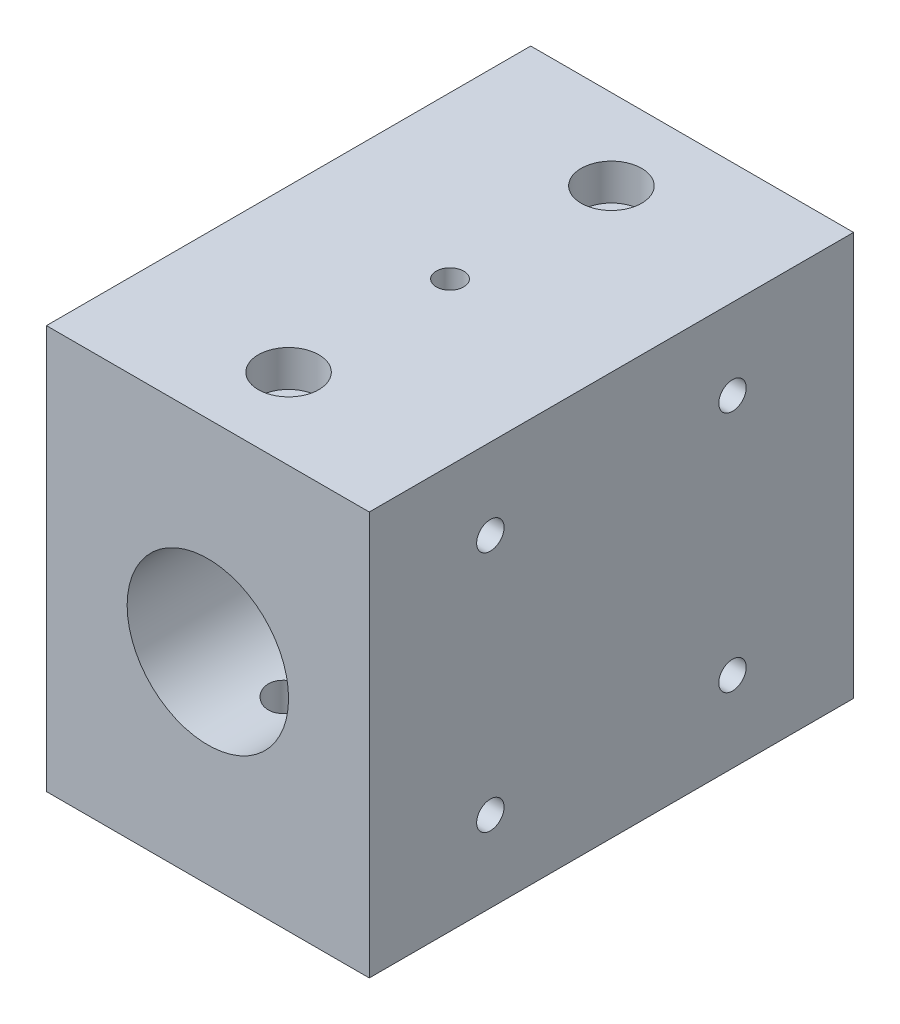
SolidWorks part; units mm, degrees
material "45#"
ref_plane "Front Plane" through (0, 0, 0) normal (0, 0, 1) x (1, 0, 0)
ref_plane "Top Plane" through (0, 0, 0) normal (0, 1, 0) x (1, 0, 0)
ref_plane "Right Plane" through (0, 0, 0) normal (1, 0, 0) x (0, 0, -1)
sketch "Sketch1" plane through (0, 0, 0) normal (0, 0, 1) x (1, 0, 0)
  line L5 (-40, 50) -> (40, 50)
  line L6 (-40, 50) -> (-40, -50)
  line L7 (-40, -50) -> (40, -50)
  line L8 (40, 50) -> (40, -50)
  line L9 (-40, 50) -> (40, -50) construction
  line L10 (-40, -50) -> (40, 50) construction
  point P0 (0, 0)
  dimension "D1" = 80
  dimension "D2" = 100
extrude "Boss-Extrude1" add sketch "Sketch1" along normal blind 120
sketch "Sketch2" plane through (0, 0, 120) normal (0, 0, 1) x (1, 0, 0)
  circle A0 centre (0, 0) radius 20
  dimension "D1" = 40
extrude "Cut-Extrude1" cut sketch "Sketch2" against normal through all
sketch "Sketch15" plane through (0, 0, 0) normal (0, 0, -1) x (-1, 0, 0)
  line L0 (-17.8606, 9) -> (-17.8606, -9)
  line L1 (0, 0) -> (0, -20) construction
  line L3 (0, 0) -> (20, 0) construction
  line L5 (17.8606, 9) -> (17.8606, -9)
  line L6 (-9, 17.8606) -> (9, 17.8606)
  line L7 (-9, -17.8606) -> (9, -17.8606)
  arc A0 (-9, -17.8606) -> (9, -17.8606) centre (0, 0) ccw
  circle A1 centre (0, 0) radius 20 construction
  arc A2 (-17.8606, 9) -> (-17.8606, -9) centre (0, 0) ccw
  arc A3 (9, 17.8606) -> (-9, 17.8606) centre (0, 0) ccw
  arc A4 (17.8606, -9) -> (17.8606, 9) centre (0, 0) ccw
  dimension "D1" = 18
extrude "Boss-Extrude2" [suppressed] add sketch "Sketch15" against normal blind 120
hole_wizard "Hole Size (based on) hex socket cap screw type 2" positions "Sketch3" profile "Sketch4" counterbore size "M8" standard "GB"
sketch "Sketch3" plane through (0, 50, 0) normal (0, 1, 0) x (1, 0, 0)
  line L0 (0, 0) -> (0, -20) construction
  point P0 (0, -20)
  point P2 (0, -100)
  dimension "D1" = 20
  dimension "D2" = 80
sketch "Sketch4" plane through (0, 50, 20) normal (1, 0, 0) x (0, 0, 1)
  line L0 (0, 0) -> (0, 38.0043)
  line L1 (0, 38.0043) -> (5, 35)
  line L2 (5, 35) -> (5, 9)
  line L3 (5, 9) -> (7.5, 9)
  line L4 (7.5, 9) -> (7.5, 0)
  line L5 (7.5, 0) -> (0, 0)
  line L10 (0, 38.0043) -> (-5, 35) construction
  line L11 (0, -6.35) -> (0, 107.95) construction
  dimension "孔直径" = 10
  dimension "孔深度" = 35
  dimension "柱形沉头孔直径" = 15
  dimension "柱形沉头孔深度" = 9
  dimension "导头角度" = 118
hole_wizard "打孔尺寸(%根据)内六角圆柱头螺钉的类型2" positions "Sketch6" profile "Sketch7" counterbore size "M8" standard "GB"
sketch "Sketch6" plane through (0, -50, 0) normal (0, -1, 0) x (-1, 0, 0)
  point P0 (0, -20)
  point P3 (0, -100)
sketch "Sketch7" plane through (0, -50, 20) normal (1, 0, 0) x (0, 0, -1)
  line L0 (0, 0) -> (0, 53.0043)
  line L1 (0, 53.0043) -> (5, 50)
  line L2 (5, 50) -> (5, 9)
  line L3 (5, 9) -> (7.5, 9)
  line L4 (7.5, 9) -> (7.5, 0)
  line L5 (7.5, 0) -> (0, 0)
  line L10 (0, 53.0043) -> (-5, 50) construction
  line L11 (0, -6.35) -> (0, 107.95) construction
  dimension "孔直径" = 10
  dimension "孔深度" = 50
  dimension "柱形沉头孔直径" = 15
  dimension "柱形沉头孔深度" = 9
  dimension "导头角度" = 118
hole_wizard "M8 Tapped Hole1" positions "Sketch8" profile "Sketch9" tap size "M8" standard "GB"
sketch "Sketch8" plane through (-40, 0, 0) normal (-1, 0, 0) x (0, 0, 1)
  line L0 (0, 0) -> (41.0233, 0) construction
  line L2 (60, 50) -> (60, 32.9358) construction
  line L3 (120, 50) -> (0, 50) construction
  point P0 (30, 30)
  point P2 (90, 30)
  point P4 (90, -30)
  point P6 (30, -30)
  dimension "D1" = 60
  dimension "D2" = 60
sketch "Sketch9" plane through (-40, 30, 30) normal (0, 1, 0) x (0, 0, 1)
  line L0 (0, 0) -> (0, 32.0429)
  line L1 (0, 32.0429) -> (3.4, 30)
  line L2 (3.4, 30) -> (3.4, 0)
  line L5 (3.4, 0) -> (0, 0)
  line L10 (0, 32.0429) -> (-3.4, 30) construction
  line L11 (0, -6.35) -> (0, 107.95) construction
  dimension "螺纹孔钻头直径" = 6.8
  dimension "螺纹孔钻头深度" = 30
  dimension "导头角度" = 118
cosmetic thread "Cosmetic Thread1" parameters "D1"=16, "D2"=8
cosmetic thread "Cosmetic Thread2" parameters "D1"=16, "D2"=8
cosmetic thread "Cosmetic Thread3" parameters "D1"=16, "D2"=8
cosmetic thread "Cosmetic Thread4" parameters "D1"=16, "D2"=8
hole_wizard "M8 Tapped Hole2" positions "Sketch10" profile "Sketch11" tap size "M8" standard "GB"
sketch "Sketch10" plane through (40, 0, 0) normal (1, 0, 0) x (0, 0, -1)
  point P0 (-90, 30)
  point P2 (-30, 30)
  point P5 (-30, -30)
  point P8 (-90, -30)
sketch "Sketch11" plane through (40, 30, 90) normal (0, 1, 0) x (0, 0, -1)
  line L0 (0, 0) -> (0, 32.0429)
  line L1 (0, 32.0429) -> (3.4, 30)
  line L2 (3.4, 30) -> (3.4, 0)
  line L5 (3.4, 0) -> (0, 0)
  line L10 (0, 32.0429) -> (-3.4, 30) construction
  line L11 (0, -6.35) -> (0, 107.95) construction
  dimension "螺纹孔钻头直径" = 6.8
  dimension "螺纹孔钻头深度" = 30
  dimension "导头角度" = 118
cosmetic thread "Cosmetic Thread5" parameters "D1"=16, "D2"=8
cosmetic thread "Cosmetic Thread6" parameters "D1"=16, "D2"=8
cosmetic thread "Cosmetic Thread7" parameters "D1"=16, "D2"=8
cosmetic thread "Cosmetic Thread8" parameters "D1"=16, "D2"=8
hole_wizard "M8 Tapped Hole3" positions "Sketch12" profile "Sketch13" tap size "M8" standard "GB"
sketch "Sketch12" plane through (0, 50, 0) normal (0, 1, 0) x (1, 0, 0)
  line L0 (-40, -60) -> (40, -60) construction
  line L1 (-40, -120) -> (-40, 0) construction
  line L2 (40, -120) -> (40, 0) construction
  point P0 (0, -60)
sketch "Sketch13" plane through (0, 50, 60) normal (1, 0, 0) x (0, 0, 1)
  line L0 (0, 0) -> (0, 47.0429)
  line L1 (0, 47.0429) -> (3.4, 45)
  line L2 (3.4, 45) -> (3.4, 0)
  line L5 (3.4, 0) -> (0, 0)
  line L10 (0, 47.0429) -> (-3.4, 45) construction
  line L11 (0, -6.35) -> (0, 107.95) construction
  dimension "螺纹孔钻头直径" = 6.8
  dimension "螺纹孔钻头深度" = 45
  dimension "导头角度" = 118
cosmetic thread "Cosmetic Thread9" parameters "D1"=16, "D2"=8
sketch "Sketch16" [suppressed] plane through (0, 0, 0) normal (0, 0, -1) x (-1, 0, 0)
  line L0 (-40, -50) -> (-40, 50) construction
  line L1 (-40, 11) -> (-30.6216, 11)
  line L2 (-40, 11) -> (-40, -11)
  line L3 (-40, -11) -> (-30.6216, -11)
  line L4 (-30.6216, 11) -> (-30.6216, -11)
  line L5 (0, 0) -> (-30.6216, 0) construction
  line L6 (0, 0) -> (0, 18.4676) construction
  line L7 (30.6216, 11) -> (30.6216, -11)
  line L8 (40, -11) -> (30.6216, -11)
  line L9 (40, 11) -> (40, -11)
  line L10 (40, 11) -> (30.6216, 11)
  line L11 (-20.6216, -9) -> (-20.6216, 9) construction
  dimension "D1" = 22
  dimension "D2" = 10
extrude "Cut-Extrude2" [suppressed] cut sketch "Sketch16" against normal through all
sketch "Sketch17" plane through (0, 0, 0) normal (0, 0, -1) x (-1, 0, 0)
  line L1 (-78.9072, 0.25) -> (78.9072, 0.25)
  line L2 (-78.9072, 0.25) -> (-78.9072, -0.25)
  line L3 (-78.9072, -0.25) -> (78.9072, -0.25)
  line L4 (78.9072, 0.25) -> (78.9072, -0.25)
  line L5 (-78.9072, 0.25) -> (78.9072, -0.25) construction
  line L6 (-78.9072, -0.25) -> (78.9072, 0.25) construction
  point P0 (0, 0)
  dimension "D1" = 0.5
extrude "Cut-Extrude3" [suppressed] cut sketch "Sketch17" against normal through all and the other way through all
